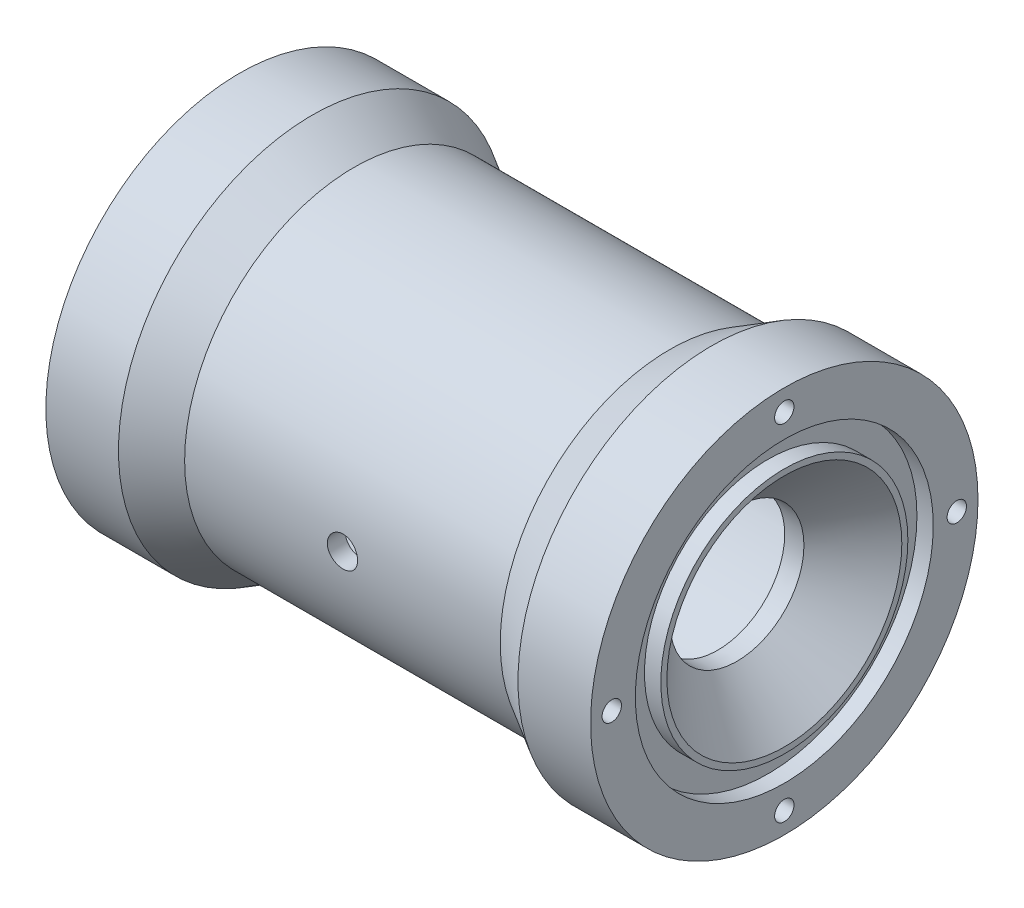
from build123d import *

# Parameters (mm, degrees)
HOLE_WIZARD_M2_1_D     = 1.6
HOLE_WIZARD_M2_1_DEPTH = 5
HOLE_WIZARD_M2_1_TIP   = 0.480688495
HOLE_WIZARD_M2_2_D     = 1.6
HOLE_WIZARD_M2_2_DEPTH = 5.2
HOLE_WIZARD_M2_2_TIP   = 0.480688495
SKETCH_9_R             = 1.25
CUT_EXTRUDE_1_DEPTH    = 20


with BuildPart() as part:
    # 草图1 → 旋转1 (revolve)
    with BuildSketch(Plane.XY, mode=Mode.PRIVATE) as revolve_1_sk:
        Polygon((16.5, 16), (13.035898385, 14), (-13.035898385, 14), (-16.5, 16), (-22.5, 16), (-22.5, 12.5), (17.00000944, 12.5), (17.004829984, 5.52730985), (18.592329605, 5.528407362), (22.501943889, 9.703811257), (22.501598217, 10.203809753), (21.151391042, 10.203809753), (21.151391042, 12.303809753), (22.497591042, 12.303809753), (22.497591042, 16), align=None)
    revolve(revolve_1_sk.sketch.rotate(Axis((22.5, 0, 0), (-1, 0, 0)), 90), axis=Axis((22.5, 0, 0), (-1, 0, 0)))

    # M2 螺纹孔1
    with Locations(Plane(origin=(22.497591042, 0, 0), x_dir=(0, 0, -1), z_dir=(1, 0, 0))):
        with Locations((0, 14.25), (14.25, 0), (0, -14.25), (-14.25, 0), (0, 0)):
            Hole(HOLE_WIZARD_M2_1_D / 2, depth=HOLE_WIZARD_M2_1_DEPTH)
            with Locations((0, 0, -(HOLE_WIZARD_M2_1_DEPTH + HOLE_WIZARD_M2_1_TIP / 2))):  # 118° drill point
                Cone(0, HOLE_WIZARD_M2_1_D / 2, HOLE_WIZARD_M2_1_TIP, mode=Mode.SUBTRACT)

    # M2 螺纹孔2
    with Locations(Plane.ZY.offset(22.5)):
        with Locations((0, 14.25), (14.25, 0), (0, -14.25), (-14.25, 0), (0, 0)):
            Hole(HOLE_WIZARD_M2_2_D / 2, depth=HOLE_WIZARD_M2_2_DEPTH)
            with Locations((0, 0, -(HOLE_WIZARD_M2_2_DEPTH + HOLE_WIZARD_M2_2_TIP / 2))):  # 118° drill point
                Cone(0, HOLE_WIZARD_M2_2_D / 2, HOLE_WIZARD_M2_2_TIP, mode=Mode.SUBTRACT)

    # 草图9 → 切除-拉伸1 (cut)
    with BuildSketch(Plane.XY):
        with Locations(Location((0, 0, 0), (0, 0, 180))):
            Circle(SKETCH_9_R)
    extrude(amount=CUT_EXTRUDE_1_DEPTH, mode=Mode.SUBTRACT)


solid = part.part
